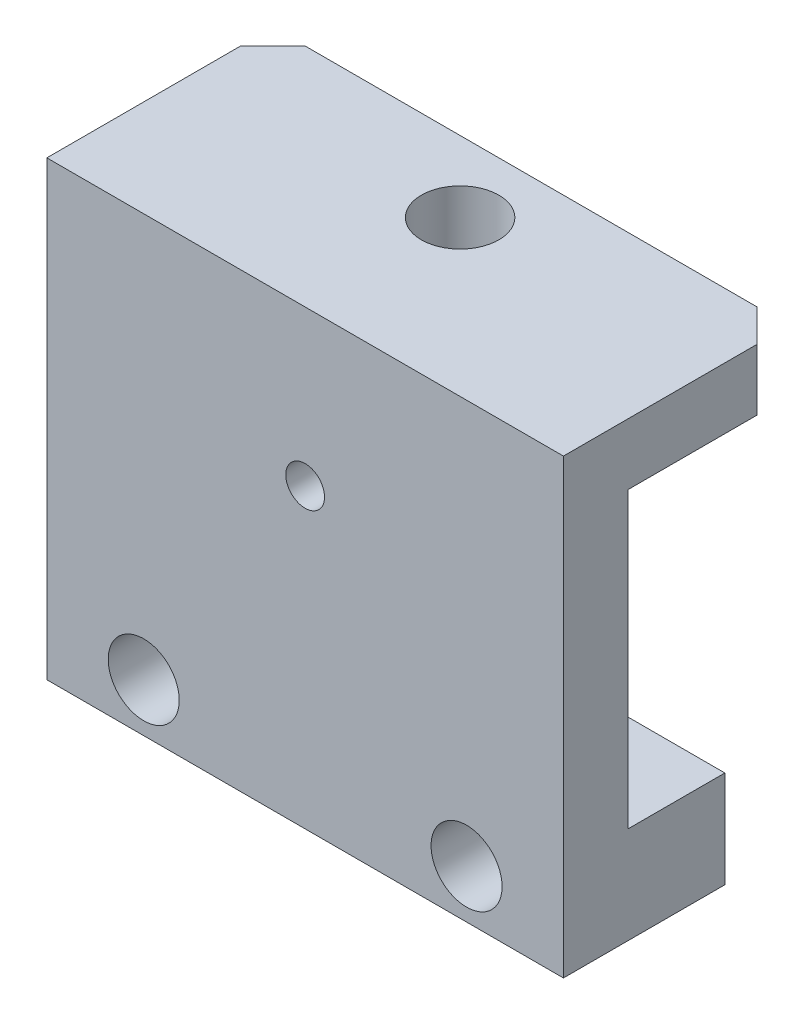
SolidWorks part; units mm, degrees
ref_plane "前视基准面" through (0, 0, 0) normal (0, 0, 1) x (1, 0, 0)
ref_plane "上视基准面" through (0, 0, 0) normal (0, 1, 0) x (1, 0, 0)
ref_plane "右视基准面" through (0, 0, 0) normal (1, 0, 0) x (0, 0, -1)
sketch "草图1" plane through (0, 0, 0) normal (0, 0, 1) x (1, 0, 0)
  line L1 (0, 0) -> (80, 0)
  line L2 (0, 0) -> (0, 70)
  line L3 (0, 70) -> (80, 70)
  line L4 (80, 0) -> (80, 70)
  dimension "D1" = 80
  dimension "D2" = 70
extrude "凸台-拉伸1" add sketch "草图1" along normal blind 25
sketch "草图2" plane through (80, 0, 0) normal (1, 0, 0) x (0, 0, -1)
  line L0 (0, 0) -> (0, 70) construction
  line L1 (-15, 60.5) -> (0, 60.5)
  line L2 (-15, 60.5) -> (-15, 15)
  line L3 (-15, 15) -> (0, 15)
  line L4 (0, 60.5) -> (0, 15)
  line L5 (-25, 0) -> (0, 0) construction
  line L6 (-25, 0) -> (-25, 70) construction
  line L7 (-25, 70) -> (0, 70) construction
  dimension "D1" = 15
  dimension "D2" = 10
  dimension "D3" = 9.5
extrude "切除-拉伸1" cut sketch "草图2" against normal blind 109
hole_wizard "M6 六角凹头螺钉的柱形沉头孔1" positions "草图6" profile "草图5" counterbore size "M6" standard "ISO" end condition through all
sketch "草图6" plane through (0, 0, 25) normal (0, 0, 1) x (1, 0, 0)
  line L0 (40, 0) -> (40, 70) construction
  line L1 (0, 0) -> (80, 0) construction
  line L2 (80, 70) -> (0, 70) construction
  point P0 (15, 7.5)
  point P2 (65, 7.5)
  dimension "D1" = 50
  dimension "D2" = 7.5
sketch "草图5" plane through (15, 7.5, 25) normal (1, 0, 0) x (0, -1, 0)
  line L0 (0, 0) -> (0, 25)
  line L1 (0, 25) -> (3.2, 25)
  line L3 (3.2, 25) -> (3.2, 6.4)
  line L4 (3.2, 6.4) -> (5.5, 6.4)
  line L5 (5.5, 6.4) -> (5.5, 0)
  line L7 (5.5, 0) -> (0, 0)
  line L11 (0, -6.35) -> (0, 107.95) construction
  dimension "通孔孔直径" = 6.4
  dimension "通孔孔深度" = 25
  dimension "柱形沉头孔直径" = 11
  dimension "柱形沉头孔深度" = 6.4
sketch "草图7" plane through (0, 0, 18.6) normal (0, 0, 1) x (1, 0, 0)
  circle A0 centre (15, 7.5) radius 5.5 construction
  circle A1 centre (65, 7.5) radius 5.5 construction
  circle A2 centre (15, 7.5) radius 5.5
  circle A3 centre (65, 7.5) radius 5.5
extrude "切除-拉伸3" cut sketch "草图7" against normal blind 10
sketch "草图8" plane through (0, 0, 25) normal (0, 0, 1) x (1, 0, 0)
  line L0 (40, 0) -> (40, 70) construction
  line L1 (0, 0) -> (80, 0) construction
  line L2 (80, 70) -> (0, 70) construction
  circle A0 centre (40, 46) radius 3
  dimension "D1" = 6
  dimension "D2" = 46
extrude "切除-拉伸4" cut sketch "草图8" against normal blind 10
sketch "草图9" plane through (0, 0, 0) normal (0, 0, -1) x (-1, 0, 0)
  line L4 (-80, 60.5) -> (0, 60.5)
  line L5 (0, 60.5) -> (0, 70)
  line L6 (0, 70) -> (-80, 70)
  line L7 (-80, 70) -> (-80, 60.5)
  line L8 (-80, 60.5) -> (0, 60.5)
  line L9 (0, 60.5) -> (0, 70)
  line L10 (0, 70) -> (-80, 70)
  line L11 (-80, 70) -> (-80, 60.5)
  dimension "D1" = 0
extrude "凸台-拉伸2" add sketch "草图9" along normal blind 10
sketch "草图10" plane through (0, 70, 0) normal (0, 1, 0) x (1, 0, 0)
  line L0 (40, -25) -> (40, 15.4366) construction
  line L1 (80, -25) -> (0, -25) construction
  line L2 (0, 10) -> (80, 10) construction
  circle A0 centre (40, -1) radius 6
  dimension "D1" = 12
  dimension "D2" = 11
extrude "切除-拉伸5" cut sketch "草图10" against normal up to surface (9.5 mm away) up to face at (40, 60.5, 2.5)
chamfer "倒角1" distance 5 angle 45 2 edges at (0, 65.25, -10) (80, 65.25, -10)
